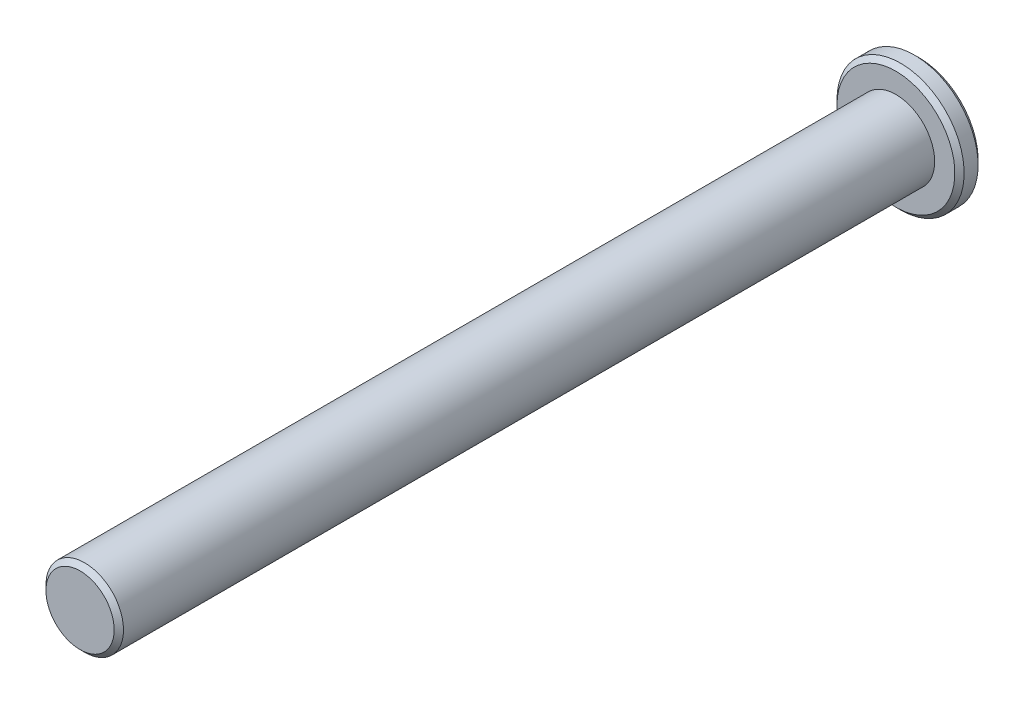
SolidWorks part; units mm, degrees
ref_plane "Front Plane" through (0, 0, 0) normal (0, 0, 1) x (1, 0, 0)
ref_plane "Top Plane" through (0, 0, 0) normal (0, 1, 0) x (1, 0, 0)
ref_plane "Right Plane" through (0, 0, 0) normal (1, 0, 0) x (0, 0, -1)
other "Configuration Table"
sketch "Sketch1" plane through (0, 0, 0) normal (0, 0, 1) x (1, 0, 0)
  circle A0 centre (0, 0) radius 25
  dimension "D1" = 50
extrude "Boss-Extrude1" add sketch "Sketch1" along normal blind 526
sketch "Sketch2" plane through (0, 0, 0) normal (0, 0, -1) x (-1, 0, 0)
  circle A0 centre (0, 0) radius 41
  dimension "D1" = 82
extrude "Boss-Extrude2" add sketch "Sketch2" along normal blind 15
chamfer "Chamfer1" distance 3 angle 45 3 edges at (-41, 0, 0) (-41, 0, -15) (25, 0, 526)
